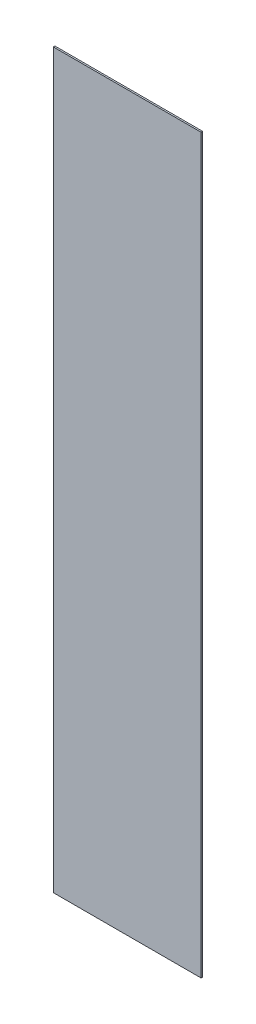
from build123d import *

# Parameters (mm, degrees)
SKETCH_1_W      = 466
SKETCH_1_H      = 2310
EXTRUDE_1_DEPTH = 5


with BuildPart() as part:
    # 草图1 → 凸台-拉伸1 (new body)
    with BuildSketch(Plane.XY):
        Rectangle(SKETCH_1_W, SKETCH_1_H)
    extrude(amount=EXTRUDE_1_DEPTH)


solid = part.part
